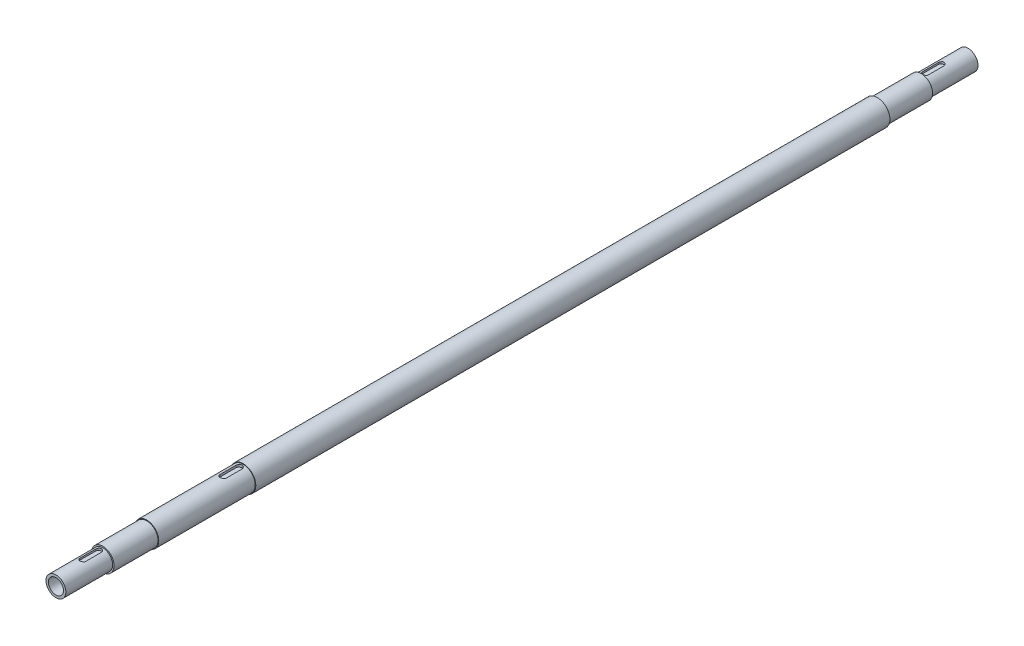
SolidWorks part; units mm, degrees
material "普通碳钢"
ref_plane "Front Plane" through (0, 0, 0) normal (0, 0, 1) x (1, 0, 0)
ref_plane "Top Plane" through (0, 0, 0) normal (0, 1, 0) x (1, 0, 0)
ref_plane "Right Plane" through (0, 0, 0) normal (1, 0, 0) x (0, 0, -1)
other "Configuration Table"
sketch "Sketch1" plane through (0, 0, 0) normal (0, 0, 1) x (1, 0, 0)
  circle A0 centre (0, 0) radius 44.5
  dimension "D1" = 89
extrude "Boss-Extrude1" add sketch "Sketch1" along normal blind 3215
sketch "Sketch2" plane through (0, 0, 3215) normal (0, 0, 1) x (1, 0, 0)
  circle A0 centre (0, 0) radius 37.5
  circle A2 centre (0, 0) radius 44.5
  dimension "D1" = 75
  dimension "D2" = 89
extrude "Cut-Extrude1" cut sketch "Sketch2" against normal blind 165
sketch "Sketch3" plane through (0, 0, 3050) normal (0, 0, 1) x (1, 0, 0)
  circle A0 centre (0, 0) radius 40
  circle A1 centre (0, 0) radius 44.5
  dimension "D1" = 80
  dimension "D2" = 89
extrude "Cut-Extrude2" cut sketch "Sketch3" against normal blind 155
sketch "Sketch4" plane through (0, 0, 2895) normal (0, 0, 1) x (1, 0, 0)
  circle A0 centre (0, 0) radius 42.5
  circle A1 centre (0, 0) radius 44.5
  dimension "D1" = 85
  dimension "D2" = 89
extrude "Cut-Extrude3" cut sketch "Sketch4" against normal blind 340
sketch "Sketch5" plane through (0, 0, 2555) normal (0, 0, 1) x (1, 0, 0)
  circle A0 centre (0, 0) radius 35
  circle A1 centre (0, 0) radius 38
  dimension "D1" = 70
  dimension "D2" = 76
ref_plane "Plane1" through (0, 40, 0) normal (0, 1, 0) x (1, 0, 0)
sketch "Sketch6" plane through (0, 40, 0) normal (0, 1, 0) x (1, 0, 0)
  line L0 (0, -2907.5) -> (0, -3050) construction
  line L1 (12.5, -2907.5) -> (12.5, -3050)
  line L2 (-12.5, -2907.5) -> (-12.5, -3050)
  line L3 (-37.5, -3050) -> (37.5, -3050) construction
  line L4 (-12.5, -3050) -> (12.5, -3050)
  arc A0 (12.5, -2907.5) -> (-12.5, -2907.5) centre (0, -2907.5) ccw
  point P2 (0, -2929)
  dimension "D2" = 142.5
  dimension "D3" = 142.5
  dimension "D4" = 12.5
  dimension "D1" = 25
  dimension "D5" = 25
extrude "Cut-Extrude5" [suppressed] cut sketch "Sketch6" against normal blind 9
sketch "Sketch7" plane through (0, 40, 0) normal (0, 1, 0) x (1, 0, 0)
  line L0 (0, -2445) -> (0, -2535) construction
  line L1 (12.5, -2445) -> (12.5, -2535)
  line L2 (-12.5, -2445) -> (-12.5, -2535)
  line L4 (-42.5, -2555) -> (42.5, -2555) construction
  arc A0 (12.5, -2445) -> (-12.5, -2445) centre (0, -2445) ccw
  arc A1 (-12.5, -2535) -> (12.5, -2535) centre (0, -2535) ccw
  point P3 (0, -2490)
  dimension "D1" = 25
  dimension "D2" = 90
  dimension "D3" = 20
extrude "Cut-Extrude6" [suppressed] cut sketch "Sketch7" against normal blind 9
ref_plane "Plane2" through (0, 0, 1607.5) normal (0, 0, 1) x (1, 0, 0)
sketch "Sketch8" plane through (0, 0, 3215) normal (0, 0, 1) x (1, 0, 0)
  circle A0 centre (0, 0) radius 26.5
  dimension "D1" = 53
extrude "Cut-Extrude7" cut sketch "Sketch8" against normal through all
sketch "Sketch9" plane through (0, 0, 3215) normal (0, 0, 1) x (1, 0, 0)
  circle A0 centre (0, 0) radius 27.5
  circle A1 centre (0, 0) radius 38
  dimension "D1" = 76
  dimension "D2" = 55
sketch "Sketch10" plane through (0, 0, 3215) normal (0, 0, 1) x (1, 0, 0)
  circle A0 centre (0, 0) radius 35
  circle A1 centre (0, 0) radius 37.5
  dimension "D1" = 70
  dimension "D2" = 75
extrude "Cut-Extrude8" cut sketch "Sketch10" against normal up to surface (165 mm away) up to face at (37.5, 0, 3050)
mirror "Mirror1" about plane through (0, 0, 1607.5) normal (0, 0, 1) of "Cut-Extrude8", "Cut-Extrude1", "Cut-Extrude2", "Cut-Extrude5"
chamfer "Chamfer1" [suppressed] distance 1 angle 45
ref_plane "Plane3" through (0, 35, 0) normal (0, 1, 0) x (1, 0, 0)
sketch "Sketch11" plane through (0, 35, 0) normal (0, 1, 0) x (1, 0, 0)
  line L0 (0, -3065) -> (0, -3050) construction
  line L1 (10, -3065) -> (10, -3120)
  line L2 (-10, -3065) -> (-10, -3120)
  line L3 (-35, -3050) -> (35, -3050) construction
  line L5 (-35, -3050) -> (35, -3050) construction
  line L7 (10, -3120) -> (-10, -3120) construction
  arc A0 (10, -3065) -> (-10, -3065) centre (0, -3065) ccw
  arc A2 (-10, -3120) -> (10, -3120) centre (0, -3120) ccw
  point P3 (0, -3120)
  dimension "D4" = 10
  dimension "D2" = 15
  dimension "D1" = 20
  dimension "D3" = 55
extrude "Cut-Extrude9" cut sketch "Sketch11" against normal blind 7.5
mirror "Mirror2" about plane through (0, 0, 1607.5) normal (0, 0, 1) of "Cut-Extrude9"
ref_plane "Plane4" through (0, 42.5, 0) normal (0, 1, 0) x (1, 0, 0)
sketch "Sketch12" plane through (0, 42.5, 0) normal (0, 1, 0) x (1, 0, 0)
  line L0 (0, -2555) -> (0, -2625) construction
  line L1 (-42.5, -2555) -> (42.5, -2555) construction
  line L2 (11, -2570) -> (11, -2625)
  line L3 (-11, -2570) -> (-11, -2625)
  arc A1 (-11, -2625) -> (11, -2625) centre (0, -2625) ccw
  arc A2 (-11, -2570) -> (11, -2570) centre (0, -2570) cw
  dimension "D4" = 11
  dimension "D1" = 55
  dimension "D2" = 15
  dimension "D3" = 70
extrude "Cut-Extrude10" cut sketch "Sketch12" against normal blind 9
